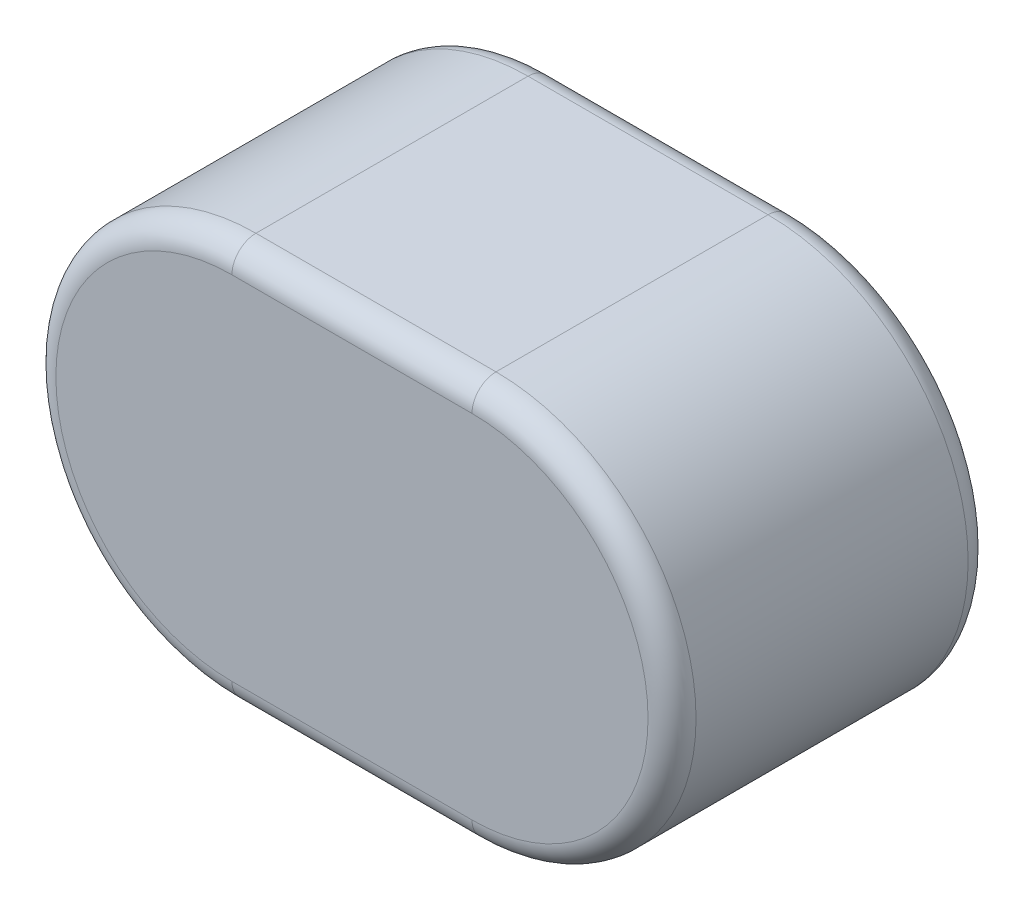
from build123d import *

# Parameters (mm, degrees)
EXTRUDE_523_DEPTH = 8
FILLET_1_R        = 0.6


with BuildPart() as part:
    # 草图1 → Extrude 523 (new body)
    with BuildSketch(Plane.XY):
        with BuildLine():
            Line((-3, 5), (3, 5))
            ThreePointArc((3, 5), (8, 0), (3, -5))
            Line((3, -5), (-3, -5))
            ThreePointArc((-3, -5), (-8, 0), (-3, 5))
        make_face()
    extrude(amount=EXTRUDE_523_DEPTH)

    # 圆角1
    fillet_1_edges = [part.edges().sort_by_distance(p)[0] for p in [
        (8, 0, 8),
        (0, 5, 8),
        (-8, 0, 8),
        (0, 5, 0),
        (8, 0, 0),
        (0, -5, 0),
        (-8, 0, 0),
        (0, -5, 8),
    ]]
    fillet(fillet_1_edges, radius=FILLET_1_R)


solid = part.part
